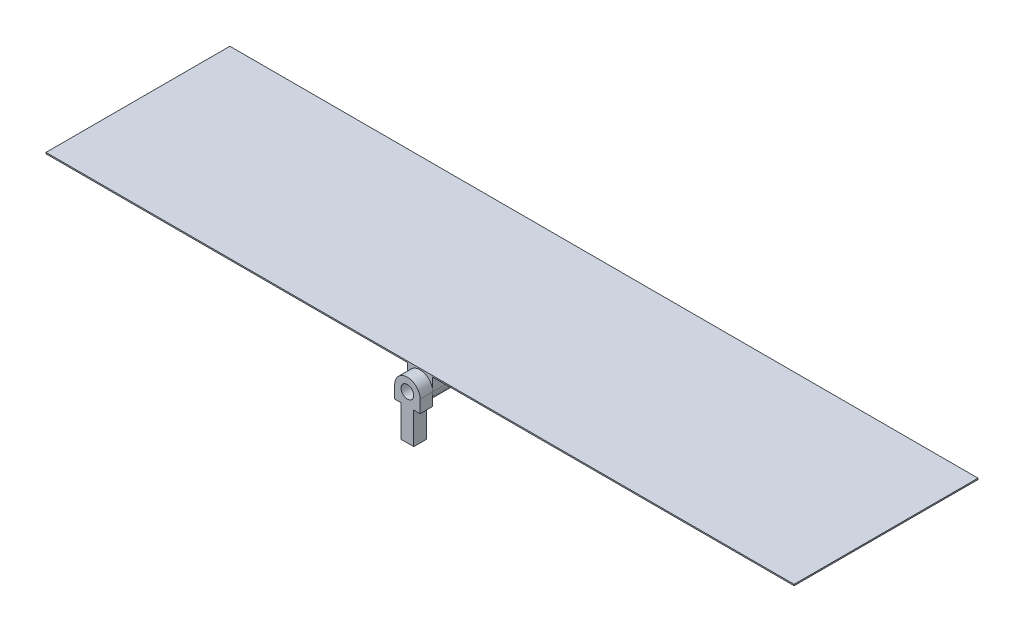
SolidWorks part; units mm, degrees
ref_plane "前视基准面" through (0, 0, 0) normal (0, 0, 1) x (1, 0, 0)
ref_plane "上视基准面" through (0, 0, 0) normal (0, 1, 0) x (1, 0, 0)
ref_plane "右视基准面" through (0, 0, 0) normal (1, 0, 0) x (0, 0, -1)
sketch "草图1" plane through (0, 0, 0) normal (0, 0, 1) x (1, 0, 0)
  line L0 (-10, 0) -> (-10, 10)
  line L1 (-10, 10) -> (10, 10)
  line L2 (10, 10) -> (10, 0)
  arc A0 (-10, 0) -> (10, 0) centre (0, 0) ccw
  circle A1 centre (0, 0) radius 5
extrude "凸台-拉伸1" add sketch "草图1" along normal mid plane 145
sketch "草图2" plane through (0, 10, 0) normal (0, 1, 0) x (1, 0, 0)
  line L0 (10, 72.5) -> (-10, 72.5) construction
  line L1 (-295, 72.5) -> (295, 72.5)
  line L2 (-295, 72.5) -> (-295, -72.5)
  line L3 (-295, -72.5) -> (295, -72.5)
  line L4 (295, 72.5) -> (295, -72.5)
  dimension "D1" = 145
  dimension "D2" = 590
  dimension "D3" = 295
extrude "凸台-拉伸2" add sketch "草图2" along normal blind 1 separate body
sketch "草图4" plane through (0, 0, 0) normal (0, 0, 1) x (1, 0, 0)
  line L1 (-10, 10) -> (-250, 10)
  line L3 (-295, 10) -> (295, 10) construction
  line L4 (-250, 10) -> (-250, 5)
  line L5 (-250, 5) -> (-0.5996, -9.982)
  line L6 (10, 10) -> (249.9979, 11)
  line L7 (-295, 11) -> (295, 11) construction
  line L8 (249.9979, 11) -> (249.9979, 6)
  line L9 (249.9979, 6) -> (0.6395, -9.9795)
  line L10 (-10, 10) -> (-10, 0)
  line L11 (10, 0) -> (10, 10)
  arc A0 (-10, 0) -> (10, 0) centre (0, 0) ccw construction
  arc A1 (-10, 0) -> (-0.5996, -9.982) centre (0, 0) ccw
  arc A2 (0.6395, -9.9795) -> (10, 0) centre (0, 0) ccw
extrude "凸台-拉伸3" add sketch "草图4" along normal mid plane 10
sketch "草图5" plane through (0, 0, 72.5) normal (0, 0, 1) x (1, 0, 0)
  line L0 (-10, 0) -> (-10, -10)
  line L1 (5, -10) -> (10, -10)
  line L2 (10, -10) -> (10, 0)
  line L3 (-5, -10) -> (-10, -10)
  line L4 (5, -25) -> (5, -10)
  line L5 (-5, -25) -> (-5, -10)
  line L6 (-5, -25) -> (-5, -35)
  line L7 (-5, -35) -> (5, -35)
  line L8 (5, -35) -> (5, -25)
  circle A0 centre (0, 0) radius 5
  arc A1 (10, 0) -> (-10, 0) centre (0, 0) ccw
extrude "凸台-拉伸4" add sketch "草图5" along normal blind 10
